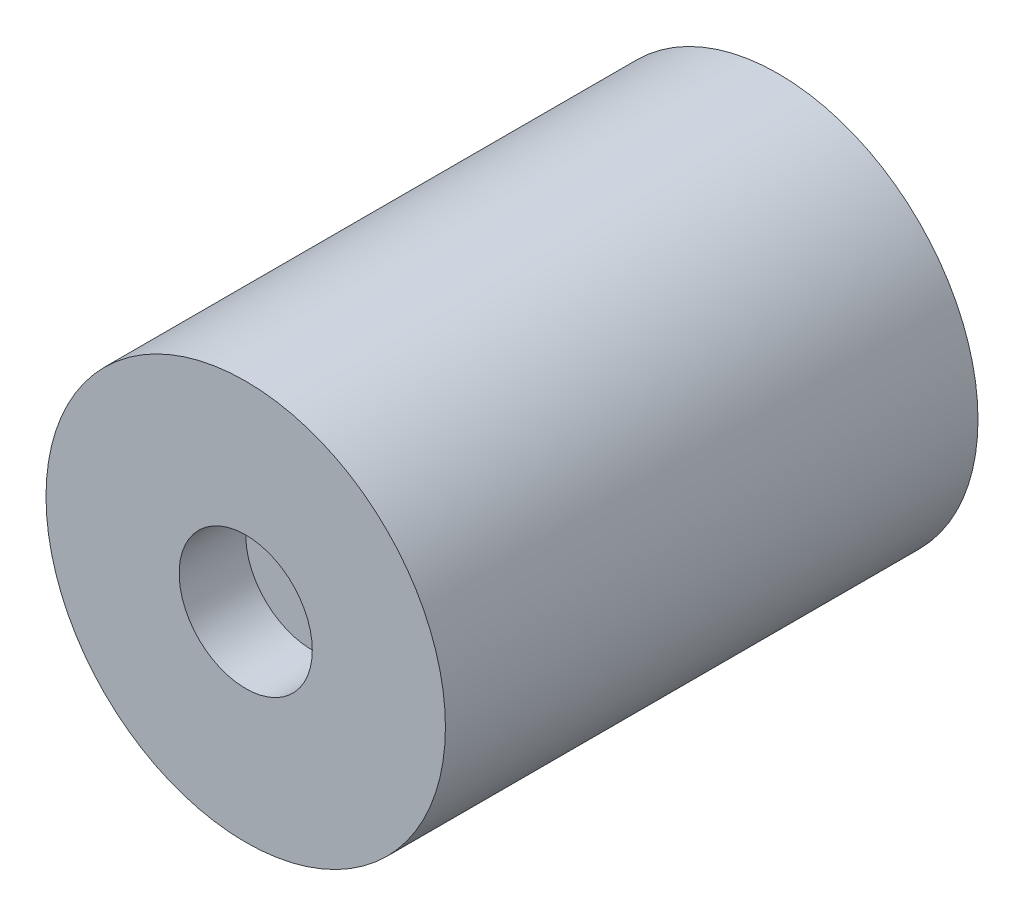
SolidWorks part; units mm, degrees
ref_plane "Front Plane" through (0, 0, 0) normal (0, 0, 1) x (1, 0, 0)
ref_plane "Top Plane" through (0, 0, 0) normal (0, 1, 0) x (1, 0, 0)
ref_plane "Right Plane" through (0, 0, 0) normal (1, 0, 0) x (0, 0, -1)
sketch "Sketch1" plane through (0, 0, 0) normal (0, 0, 1) x (1, 0, 0)
  circle A0 centre (-276.5313, -10.1177) radius 1.5
extrude "Boss-Extrude1" add sketch "Sketch1" along normal blind 4
sketch "Sketch4" plane through (0, 0, 4) normal (0, 0, 1) x (1, 0, 0)
  circle A0 centre (-276.5313, -10.1177) radius 0.5
extrude "Cut-Extrude1" cut sketch "Sketch4" against normal blind 0.5
sketch "Sketch5" plane through (0, 0, 0) normal (0, 0, -1) x (-1, 0, 0)
  circle A0 centre (276.5313, -10.1177) radius 0.5
extrude "Cut-Extrude2" cut sketch "Sketch5" against normal blind 0.25
